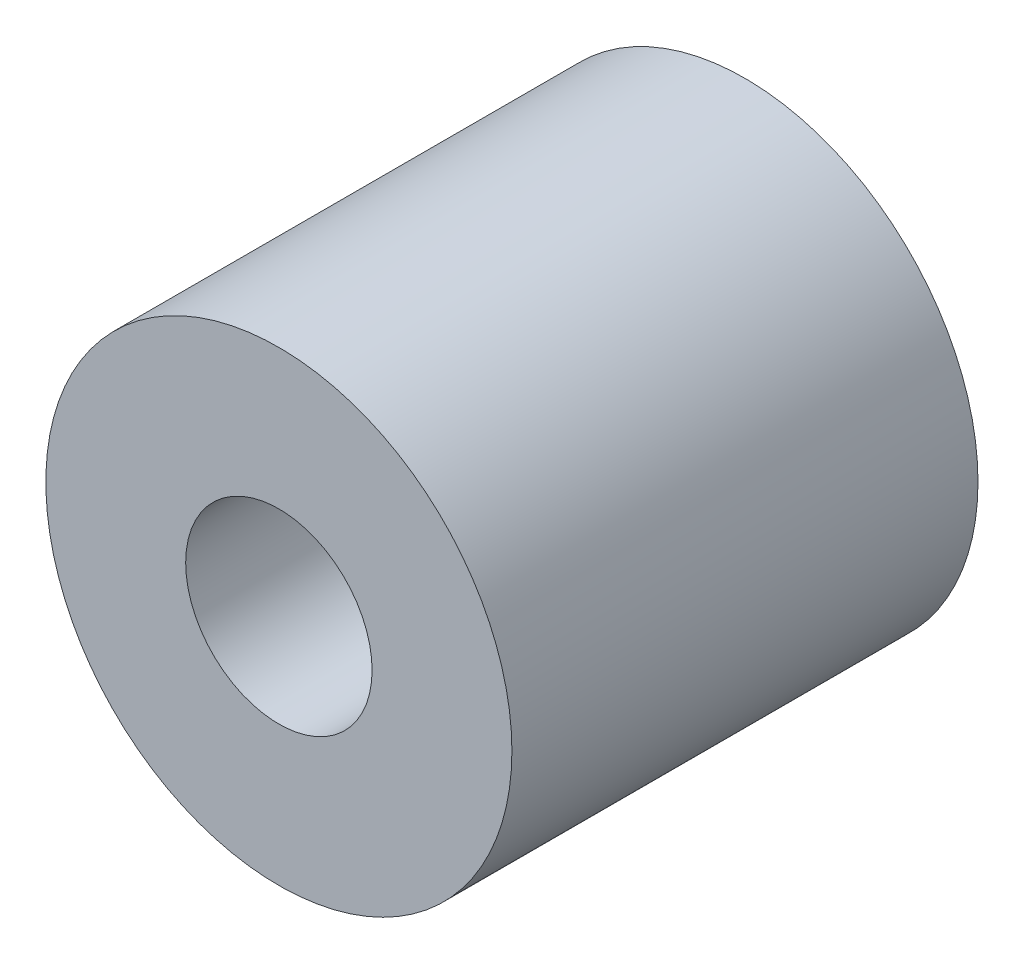
from build123d import *

# Parameters (mm, degrees)
SKETCH_1_R      = 10
SKETCH_1_R_2    = 4
EXTRUDE_1_DEPTH = 20


with BuildPart() as part:
    # 草图1 → 凸台-拉伸1 (new body)
    with BuildSketch(Plane.XY):
        Circle(SKETCH_1_R)
        Circle(SKETCH_1_R_2, mode=Mode.SUBTRACT)
    extrude(amount=EXTRUDE_1_DEPTH)


solid = part.part
